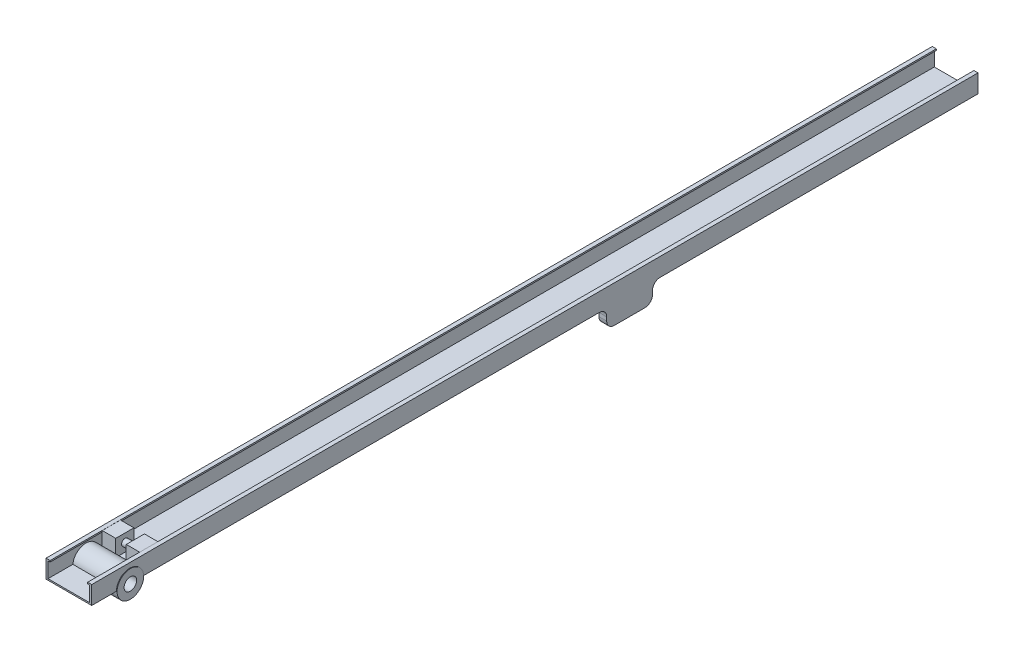
SolidWorks part; units mm, degrees
ref_plane "Front Plane" through (0, 0, 0) normal (0, 0, 1) x (1, 0, 0)
ref_plane "Top Plane" through (0, 0, 0) normal (0, 1, 0) x (1, 0, 0)
ref_plane "Right Plane" through (0, 0, 0) normal (1, 0, 0) x (0, 0, -1)
sketch "Sketch1" plane through (0, 0, 0) normal (0, 0, 1) x (1, 0, 0)
  line L0 (-300, 145) -> (-300, 122.5)
  line L1 (-365, 145) -> (-300, 145)
  line L2 (-365, 145) -> (-365, -145)
  line L3 (-365, -145) -> (365, -145)
  line L4 (365, 145) -> (365, -145)
  line L5 (300, 122.5) -> (332.5, 122.5)
  line L6 (332.5, -122.5) -> (332.5, 122.5)
  line L7 (332.5, -122.5) -> (-332.5, -122.5)
  line L10 (-332.5, -122.5) -> (-332.5, 122.5)
  line L13 (0, 145) -> (0, -311.303) construction
  line L14 (-300, 122.5) -> (-332.5, 122.5)
  line L18 (365, 145) -> (300, 145)
  line L19 (300, 145) -> (300, 122.5)
  point P0 (0, 0)
  point P6 (0, 0)
  dimension "D1" = 730
  dimension "D2" = 290
  dimension "D3" = 245
  dimension "D5" = 32.5
extrude "Boss-Extrude1" add sketch "Sketch1" along normal mid plane 14150
sketch "Sketch4" plane through (0, -145, 0) normal (0, -1, 0) x (1, 0, 0)
  line L0 (365, 7075) -> (365, -7075) construction
  line L1 (-365, -1146.9738) -> (365, -1146.9738)
  line L2 (-365, -1146.9738) -> (-365, -1878.4836)
  line L3 (-365, -1878.4836) -> (365, -1878.4836)
  line L4 (365, -1146.9738) -> (365, -1878.4836)
  line L5 (-365, -1146.9738) -> (365, -1878.4836) construction
  line L6 (-365, -1878.4836) -> (365, -1146.9738) construction
  point P0 (0, -1512.7287)
extrude "Boss-Extrude2" add sketch "Sketch4" along normal blind 299
fillet "Fillet1" radius 120 2 edges at (0, -444, -1146.9738) (0, -444, -1878.4836)
fillet "Fillet2" radius 120 2 edges at (0, -145, -1878.4836) (0, -145, -1146.9738)
sketch "Sketch7" plane through (0, 0, 0) normal (1, 0, 0) x (0, 0, -1)
  line L0 (-7075, -145) -> (1026.9738, -145) construction
  circle A0 centre (-6467.9961, -145) radius 212.1196
extrude "Boss-Extrude3" add sketch "Sketch7" along normal mid plane 750
sketch "Sketch8" plane through (0, 0, 0) normal (1, 0, 0) x (0, 0, -1)
  circle A0 centre (-6467.9961, -145) radius 87.5
  dimension "D1" = 175
extrude "Boss-Extrude4" add sketch "Sketch8" along normal mid plane 850
sketch "Sketch9" plane through (0, 0, -1146.9738) normal (0, 0, 1) x (1, 0, 0)
  line L1 (-242.06, -622.7933) -> (242.06, -622.7933)
  line L2 (-242.06, -622.7933) -> (-242.06, -141.1998)
  line L3 (-242.06, -141.1998) -> (242.06, -141.1998)
  line L4 (242.06, -622.7933) -> (242.06, -141.1998)
  line L5 (-242.06, -622.7933) -> (242.06, -141.1998) construction
  line L6 (-242.06, -141.1998) -> (242.06, -622.7933) construction
  point P0 (0, -381.9966)
extrude "Cut-Extrude1" cut sketch "Sketch9" against normal blind 930 and the other way blind 194
sketch "Sketch12" plane through (242.06, 0, 0) normal (-1, 0, 0) x (0, 0, 1)
  line L0 (-1266.9738, -444) -> (-1758.4836, -444) construction
  circle A0 centre (-1512.7287, -294) radius 85
  point P4 (-1512.7287, -444)
  dimension "D1" = 170
  dimension "D2" = 150
extrude "Boss-Extrude5" add sketch "Sketch12" along normal blind 548
sketch "Sketch14" plane through (242.06, 0, 0) normal (-1, 0, 0) x (0, 0, 1)
  circle A0 centre (-1512.7287, -294) radius 90
  dimension "D1" = 180
extrude "Boss-Extrude6" add sketch "Sketch14" along normal blind 167.01
sketch "Sketch15" plane through (-242.06, 0, 0) normal (1, 0, 0) x (0, 0, -1)
  circle A0 centre (1512.7287, -294) radius 90
  dimension "D1" = 180
extrude "Boss-Extrude7" add sketch "Sketch15" along normal blind 167.01
sketch "Sketch16" plane through (0, -122.5, 0) normal (0, 1, 0) x (1, 0, 0)
  line L1 (300, -7075) -> (300, 7075) construction
  line L2 (84, -5952.1784) -> (300, -5952.1784)
  line L3 (84, -5952.1784) -> (84, -6242.7575)
  line L4 (84, -6242.7575) -> (300, -6242.7575)
  line L5 (300, -5952.1784) -> (300, -6242.7575)
  line L6 (84, -5952.1784) -> (300, -6242.7575) construction
  line L7 (84, -6242.7575) -> (300, -5952.1784) construction
  line L8 (0, -5802.1252) -> (0, -6871.5517) construction
  line L9 (-84, -6242.7575) -> (-300, -5952.1784) construction
  line L10 (-84, -5952.1784) -> (-300, -6242.7575) construction
  line L11 (-300, -5952.1784) -> (-300, -6242.7575)
  line L12 (-84, -6242.7575) -> (-300, -6242.7575)
  line L13 (-84, -5952.1784) -> (-84, -6242.7575)
  line L14 (-84, -5952.1784) -> (-300, -5952.1784)
  point P0 (192, -6097.468)
  point P14 (-192, -6097.468)
  dimension "D1" = 168
extrude "Boss-Extrude8" add sketch "Sketch16" along normal blind 266
sketch "Sketch17" plane through (84, 0, 0) normal (-1, 0, 0) x (0, 0, 1)
  circle A0 centre (6094.7969, 15.55) radius 55
  dimension "D1" = 110
extrude "Boss-Extrude9" add sketch "Sketch17" along normal blind 238
sketch "Sketch18" plane through (425, 0, 0) normal (1, 0, 0) x (0, 0, -1)
  circle A1 centre (-6467.9961, -145) radius 87.5
  circle A2 centre (-6467.9961, -145) radius 87.5
  dimension "D1" = 0
extrude "Cut-Extrude2" cut sketch "Sketch18" against normal through all
sketch "Sketch19" plane through (375, 0, 0) normal (1, 0, 0) x (0, 0, -1)
  circle A0 centre (-6467.9961, -145) radius 100
  dimension "D1" = 200
extrude "Cut-Extrude3" cut sketch "Sketch19" against normal through all
